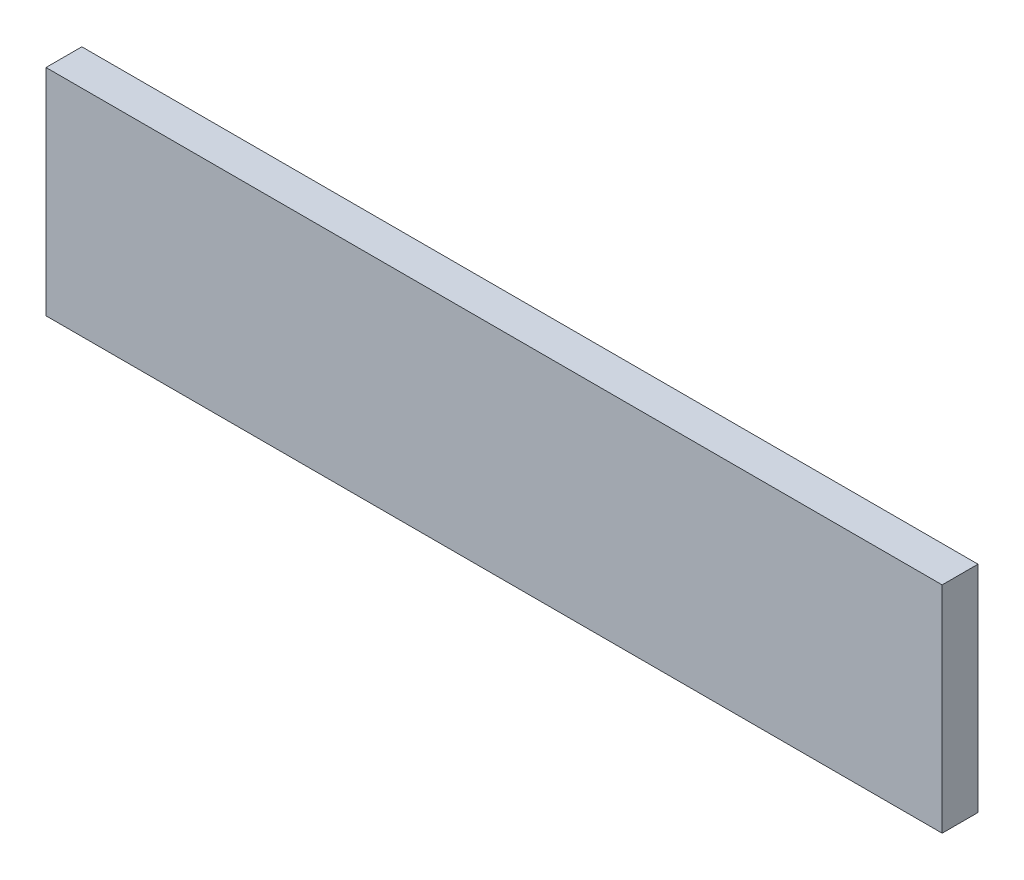
SolidWorks part; units mm, degrees
ref_plane "前视基准面" through (0, 0, 0) normal (0, 0, 1) x (1, 0, 0)
ref_plane "ZZ" through (0, 0, 0) normal (0, 1, 0) x (1, 0, 0)
ref_plane "右视基准面" through (0, 0, 0) normal (1, 0, 0) x (0, 0, -1)
sketch "草图1" plane through (0, 0, 0) normal (0, 0, 1) x (1, 0, 0)
  line L1 (625, -150) -> (-625, -150)
  line L2 (625, -150) -> (625, 150)
  line L3 (625, 150) -> (-625, 150)
  line L4 (-625, -150) -> (-625, 150)
  line L5 (625, -150) -> (-625, 150) construction
  line L6 (625, 150) -> (-625, -150) construction
  point P0 (0, 0)
  dimension "D1" = 1250
  dimension "D2" = 300
extrude "凸台-拉伸1" add sketch "草图1" along normal blind 50
